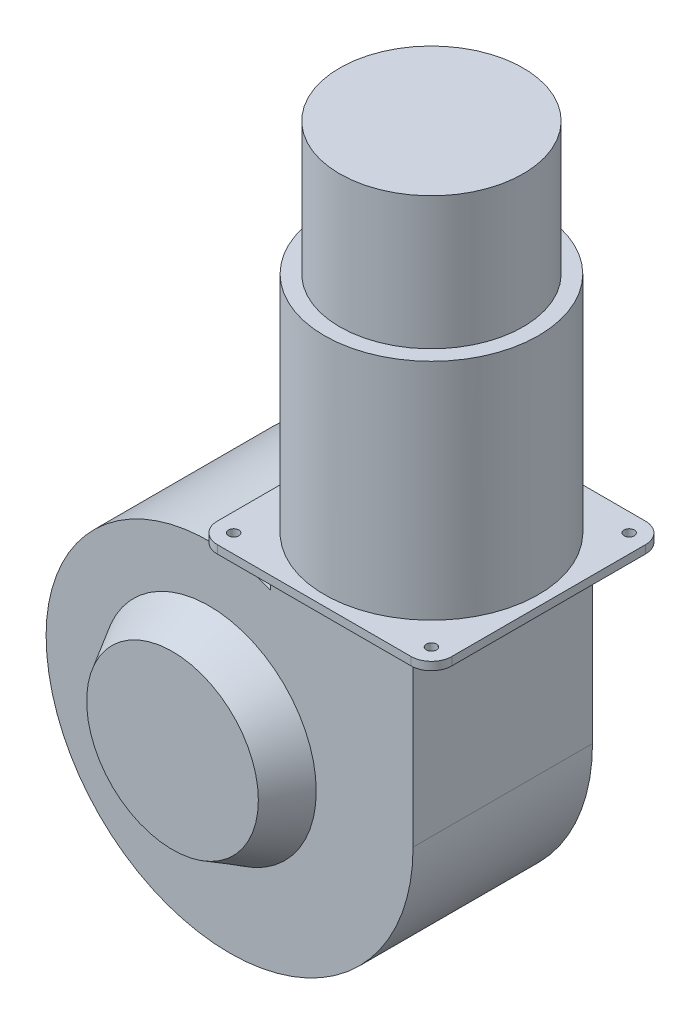
from build123d import *

# Parameters (mm, degrees)
EXTRUDE_1_DEPTH      = 88
SKETCH_2_R           = 52.5
EXTRUDE_2_DEPTH      = 18
EXTRUDE_2_TAPER      = 30
SKETCH_3_R           = 2.5
EXTRUDE_3_DEPTH      = 4
SKETCH_4_R           = 52.5
EXTRUDE_4_DEPTH      = 110
SKETCH_5_R           = 45
EXTRUDE_5_DEPTH      = 65
EXTRUDE_6_DEPTH      = 5
EXTRUDE_6_DEPTH_BACK = 5
SKETCH_7_R           = 4
EXTRUDE_7_DEPTH      = 8


with BuildPart() as part:
    # 草图1 → 凸台-拉伸1 (new body)
    with BuildSketch(Plane.XY):
        with BuildLine():
            Line((100, 0), (100, 90))
            Line((100, 90), (30, 90))
            Line((30, 90), (30, 74.161984871))
            ThreePointArc((30, 74.161984871), (-44.72135955, 66.332495807), (-80, 0))
            ThreePointArc((-80, 0), (10, -90), (100, 0))
        make_face()
    extrude(amount=EXTRUDE_1_DEPTH)

    # 草图2 → 凸台-拉伸2 (add)
    with BuildSketch(Plane.XY.offset(88)):
        Circle(SKETCH_2_R)
    extrude(amount=EXTRUDE_2_DEPTH, taper=EXTRUDE_2_TAPER)

    # 草图3 → 凸台-拉伸3 (add)
    with BuildSketch(Plane(origin=(0, 90, 0), x_dir=(1, 0, 0), z_dir=(0, 1, 0))):
        with BuildLine():
            Line((17.5, 13.5), (112.5, 13.5))
            ThreePointArc((112.5, 13.5), (119.571067812, 10.571067812), (122.5, 3.5))
            Line((122.5, 3.5), (122.5, -91.5))
            ThreePointArc((122.5, -91.5), (119.571067812, -98.571067812), (112.5, -101.5))
            Line((112.5, -101.5), (17.5, -101.5))
            ThreePointArc((17.5, -101.5), (10.428932188, -98.571067812), (7.5, -91.5))
            Line((7.5, -91.5), (7.5, 3.5))
            ThreePointArc((7.5, 3.5), (10.428932188, 10.571067812), (17.5, 13.5))
        make_face()
        with Locations(Location((16.5, 4.5, 0), (0, 0, 270))):
            Circle(SKETCH_3_R, mode=Mode.SUBTRACT)
        with Locations(Location((16.5, -92.5, 0), (0, 0, 90))):
            Circle(SKETCH_3_R, mode=Mode.SUBTRACT)
        with Locations(Location((113.5, -92.5, 0), (0, 0, 270))):
            Circle(SKETCH_3_R, mode=Mode.SUBTRACT)
        with Locations(Location((113.5, 4.5, 0), (0, 0, 90))):
            Circle(SKETCH_3_R, mode=Mode.SUBTRACT)
    extrude(amount=EXTRUDE_3_DEPTH)

    # 草图4 → 凸台-拉伸4 (add)
    with BuildSketch(Plane(origin=(0, 94, 0), x_dir=(1, 0, 0), z_dir=(0, 1, 0))):
        with Locations(Location((65, -44, 0), (0, 0, 90))):
            Circle(SKETCH_4_R)
    extrude(amount=EXTRUDE_4_DEPTH)

    # 草图5 → 凸台-拉伸5 (add)
    with BuildSketch(Plane(origin=(0, 204, 0), x_dir=(1, 0, 0), z_dir=(0, 1, 0))):
        with Locations(Location((65, -44, 0), (0, 0, 270))):
            Circle(SKETCH_5_R)
    extrude(amount=EXTRUDE_5_DEPTH)



with BuildPart() as body_2:
    # 草图6 → 凸台-拉伸6 (new, two sides: drawn at the far end of the back side and taken through both)
    with BuildSketch(Plane.ZY.offset(-20).offset(-EXTRUDE_6_DEPTH_BACK)):
        Polygon((44, 239), (39.669872981, 236.5), (39.669872981, 231.5), (44, 229), (48.330127019, 231.5), (48.330127019, 236.5), align=None)
    extrude(amount=EXTRUDE_6_DEPTH + EXTRUDE_6_DEPTH_BACK)


with BuildPart() as part_1:
    add(part.part)

    add(body_2.part)  # 凸台-拉伸7 merges body 2
    # 草图7 → 凸台-拉伸7 (add)
    with BuildSketch(Plane.ZY.offset(-15)):
        with Locations((44, 234)):
            Circle(SKETCH_7_R)
    extrude(amount=EXTRUDE_7_DEPTH)


solid = part_1.part
